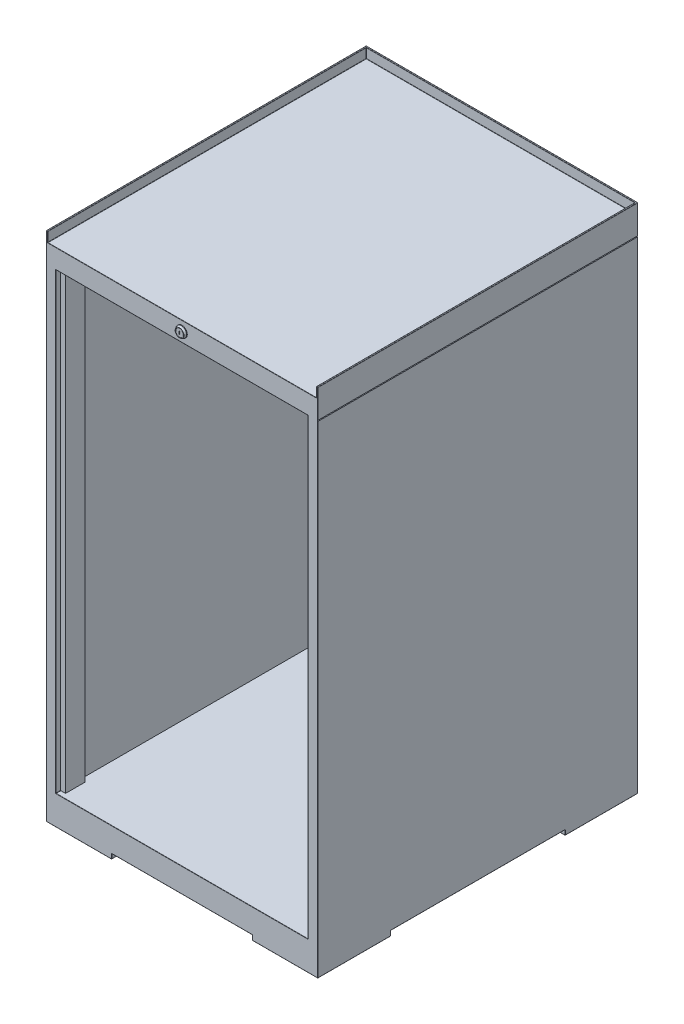
SolidWorks part; units mm, degrees
ref_plane "Frontal" through (0, 0, 0) normal (0, 0, 1) x (1, 0, 0)
ref_plane "Superior" through (0, 0, 0) normal (0, 1, 0) x (1, 0, 0)
ref_plane "Direito" through (0, 0, 0) normal (1, 0, 0) x (0, 0, -1)
sketch "Sketch1" plane through (0, 0, 0) normal (0, 0, 1) x (1, 0, 0)
  line L1 (-280, 527.5) -> (280, 527.5)
  line L2 (-280, 527.5) -> (-280, -527.5)
  line L3 (-280, -527.5) -> (280, -527.5)
  line L4 (280, 527.5) -> (280, -527.5)
  line L5 (-280, 527.5) -> (280, -527.5) construction
  line L6 (-280, -527.5) -> (280, 527.5) construction
  point P0 (0, 0)
  dimension "D1" = 560
  dimension "D2" = 1055
extrude "Boss-Extrude1" add sketch "Sketch1" along normal blind 660
sketch "Sketch2" plane through (0, 0, 660) normal (0, 0, 1) x (1, 0, 0)
  line L0 (280, 527.5) -> (-280, 527.5) construction
  line L1 (-277, 547.5) -> (277, 547.5)
  line L2 (-277, 547.5) -> (-277, 507.5)
  line L3 (-277, 507.5) -> (277, 507.5)
  line L4 (277, 547.5) -> (277, 507.5)
  line L5 (-277, 547.5) -> (277, 507.5) construction
  line L6 (-277, 507.5) -> (277, 547.5) construction
  line L7 (-280, 527.5) -> (-280, -527.5) construction
  point P0 (0, 527.5)
  dimension "D1" = 3
  dimension "D2" = 20
extrude "Cut-Extrude1" cut sketch "Sketch2" against normal blind 657
sketch "Sketch3" plane through (0, 0, 660) normal (0, 0, 1) x (1, 0, 0)
  line L0 (-277, 507.5) -> (277, 507.5) construction
  line L1 (-260, 467.5) -> (260, 467.5)
  line L2 (-260, 467.5) -> (-260, -467.5)
  line L3 (-260, -467.5) -> (260, -467.5)
  line L4 (260, 467.5) -> (260, -467.5)
  line L5 (-260, 467.5) -> (260, -467.5) construction
  line L6 (-260, -467.5) -> (260, 467.5) construction
  line L7 (-280, 527.5) -> (-280, -527.5) construction
  point P0 (0, 0)
  dimension "D1" = 40
  dimension "D2" = 20
extrude "Cut-Extrude2" cut sketch "Sketch3" against normal blind 657
sketch "Sketch4" plane through (0, -527.5, 0) normal (0, -1, 0) x (1, 0, 0)
  line L0 (-145, 660) -> (-145, 510)
  line L1 (-280, 660) -> (280, 660) construction
  line L2 (-145, 510) -> (-280, 510)
  line L3 (-280, 660) -> (-280, 0) construction
  line L4 (-280, 510) -> (-280, 150)
  line L5 (-280, 150) -> (-145, 150)
  line L6 (-145, 150) -> (-145, 0)
  line L7 (-280, 0) -> (280, 0) construction
  line L8 (-145, 0) -> (145, 0)
  line L9 (145, 0) -> (145, 150)
  line L10 (145, 150) -> (280, 150)
  line L11 (280, 660) -> (280, 0) construction
  line L12 (280, 150) -> (280, 510)
  line L13 (280, 510) -> (145, 510)
  line L14 (145, 510) -> (145, 660)
  line L15 (145, 660) -> (-145, 660)
  dimension "D1" = 135
  dimension "D2" = 150
  dimension "D3" = 150
  dimension "D4" = 135
extrude "Cut-Extrude3" cut sketch "Sketch4" against normal blind 10
fillet "Filete1" radius 1 2 edges at (278.5, 527.5, 660) (-278.5, 527.5, 660)
sketch "Sketch5" plane through (0, -467.5, 0) normal (0, 1, 0) x (1, 0, 0)
  line L0 (-260, -3) -> (-260, -660) construction
  line L1 (-260, -650) -> (-250, -650)
  line L2 (-260, -650) -> (-260, -610)
  line L3 (-260, -610) -> (-250, -610)
  line L4 (-250, -650) -> (-250, -610)
  line L5 (260, -3) -> (260, -660) construction
  line L6 (260, -650) -> (250, -650)
  line L7 (260, -650) -> (260, -610)
  line L8 (260, -610) -> (250, -610)
  line L9 (250, -650) -> (250, -610)
  line L10 (-260, -660) -> (260, -660) construction
  line L11 (-260, -3) -> (260, -3) construction
  line L12 (-260, -13) -> (-250, -13)
  line L13 (-260, -13) -> (-260, -53)
  line L14 (-260, -53) -> (-250, -53)
  line L15 (-250, -13) -> (-250, -53)
  line L16 (260, -13) -> (250, -13)
  line L17 (260, -13) -> (260, -53)
  line L18 (260, -53) -> (250, -53)
  line L19 (250, -13) -> (250, -53)
  dimension "D1" = 10
  dimension "D2" = 10
  dimension "D3" = 40
  dimension "D4" = 10
  dimension "D5" = 40
  dimension "D6" = 10
  dimension "D7" = 40
  dimension "D8" = 10
  dimension "D9" = 10
  dimension "D10" = 10
  dimension "D11" = 10
  dimension "D12" = 40
extrude "Boss-Extrude2" add sketch "Sketch5" along normal blind 935
sketch "Sketch6" plane through (0, 0, 660) normal (0, 0, 1) x (1, 0, 0)
  line L0 (279, 467.5) -> (280, 468.5)
  line L1 (280, -527.5) -> (280, 526.5) construction
  line L2 (280, 468.5) -> (280, 466.5)
  line L3 (280, 466.5) -> (279, 467.5)
  line L4 (279, 467.5) -> (280, 467.5) construction
  line L5 (-279, 467.5) -> (-280, 468.5)
  line L6 (-280, 526.5) -> (-280, -527.5) construction
  line L7 (-280, 468.5) -> (-280, 466.5)
  line L8 (-280, 466.5) -> (-279, 467.5)
  line L9 (-279, 467.5) -> (-280, 467.5) construction
  dimension "D1" = 1
  dimension "D2" = 2
  dimension "D3" = 1
extrude "Cut-Extrude4" cut sketch "Sketch6" against normal through all
sketch "Sketch7" plane through (-280, 0, 0) normal (-1, 0, 0) x (0, 0, 1)
  line L0 (0, 468.5) -> (1, 467.5)
  line L1 (0, 467.5) -> (660, 467.5) construction
  line L2 (1, 467.5) -> (0, 466.5)
  line L3 (0, 466.5) -> (0, 468.5)
  dimension "D1" = 1
extrude "Cut-Extrude5" cut sketch "Sketch7" against normal through all
sketch "Sketch9" plane through (0, 0, 660) normal (0, 0, 1) x (1, 0, 0)
  line L0 (-277, 507.5) -> (277, 507.5) construction
  circle A0 centre (0, 487.5) radius 11
  dimension "D2" = 22
  dimension "D1" = 20
extrude "Boss-Extrude3" add sketch "Sketch9" along normal blind 1.5
sketch "Sketch10" plane through (0, 0, 661.5) normal (0, 0, 1) x (1, 0, 0)
  circle A1 centre (0, 487.5) radius 11
  circle A2 centre (0, 487.5) radius 11
  dimension "D1" = 0
extrude "Boss-Extrude4" add sketch "Sketch10" along normal blind 3.5 draft 30
sketch "Sketch11" plane through (0, 0, 665) normal (0, 0, 1) x (1, 0, 0)
  circle A0 centre (0, 487.5) radius 8
  circle A1 centre (0, 487.5) radius 7.75
  dimension "D1" = 16
  dimension "D2" = 15.5
extrude "Cut-Extrude6" cut sketch "Sketch11" against normal blind 5
sketch "Sketch12" plane through (0, 0, 665) normal (0, 0, 1) x (1, 0, 0)
  line L1 (-1, 490.5) -> (1, 490.5)
  line L2 (-1, 490.5) -> (-1, 484.5)
  line L3 (-1, 484.5) -> (1, 484.5)
  line L4 (1, 490.5) -> (1, 484.5)
  line L5 (-1, 490.5) -> (1, 484.5) construction
  line L6 (-1, 484.5) -> (1, 490.5) construction
  point P0 (0, 487.5)
  dimension "D1" = 6
  dimension "D2" = 2
extrude "Cut-Extrude7" cut sketch "Sketch12" against normal blind 0.5
fillet "Filete2" radius 0.5 74 edges at (-145, -522.5, 660) (-280, -522.5, 510) (0, -517.5, 660) (-145, -522.5, 0) (0, 527.5, 3) (-212.5, -517.5, 510) (145, -517.5, 585) (280, -517.5, 330) (212.5, -517.5, 150) (-145, -517.5, 75) (280, 527.5, 329.5) (280, 527.2071, 659.7071) (277, 527.5, 331) (277, 527.2071, 659.7071) (-277, 527.5, 331) (-277, 527.2071, 659.7071) (-280, 527.5, 329.5) (-280, 527.2071, 659.7071) (-280, -527.5, 75) (-212.5, -527.5, 150) (-145, -527.5, 75) (-212.5, -527.5, 0) (212.5, -527.5, 0) (145, -527.5, 75) (212.5, -527.5, 150) (280, -527.5, 75) (280, -527.5, 585) (212.5, -527.5, 510) (145, -527.5, 585) (212.5, -527.5, 660) (-212.5, -527.5, 660) (-145, -527.5, 585) (-212.5, -527.5, 510) (-280, -527.5, 585) (-145, -522.5, 510) (-145, -517.5, 585) (145, -522.5, 660) (145, -522.5, 510) (212.5, -517.5, 510) (280, -522.5, 510) (280, -522.5, 150) (145, -522.5, 150) (145, -517.5, 75) (145, -522.5, 0) (0, -517.5, 0) (-145, -522.5, 150) (-212.5, -517.5, 150) (-280, -517.5, 330) (-280, -522.5, 150) (-280, -30.5, 0) (-280, 498, 0) (-280, -30.5, 660) (280, -30.5, 660) (280, -30.5, 0) (280, 498, 0) (0, 527.5, 0) (277, 517.5, 3) (0, 507.5, 3) (-277, 517.5, 3) (-277, 507.5, 331.5) (277, 507.5, 331.5) (280, 497.5, 660) (277, 517, 660) (0, 507.5, 660) (-277, 517, 660) (-280, 497.5, 660) (-260, 467.5, 655) (260, 467.5, 655) (260, -467.5, 655) (-260, -467.5, 655) (0, -467.5, 660) (260, 0, 660) (0, 467.5, 660) (-260, 0, 660)
hole_wizard "Tapped Hole M61" positions "Sketch18" profile "Sketch17" tap size "M6" standard "ISO"
sketch "Sketch18" plane through (0, 0, 0) normal (0, 0, -1) x (-1, 0, 0)
  point P0 (-197.25, 415)
  point P3 (-82.75, 415)
  point P6 (197.25, 415)
  point P9 (82.75, 415)
sketch "Sketch17" plane through (197.25, 415, 0) normal (1, 0, 0) x (0, 1, 0)
  line L0 (0, 0) -> (0, 18.5022)
  line L1 (0, 18.5022) -> (2.5, 17)
  line L2 (2.5, 17) -> (2.5, 0)
  line L5 (2.5, 0) -> (0, 0)
  line L10 (0, 18.5022) -> (-2.5, 17) construction
  line L11 (0, -6.35) -> (0, 107.95) construction
  dimension "Tap Drill Dia." = 5
  dimension "Tap Drill Depth" = 17
  dimension "Drill Angle" = 118
cosmetic thread "Hole Thread17" parameters "D1"=3, "D2"=6
cosmetic thread "Hole Thread18" parameters "D1"=3, "D2"=6
cosmetic thread "Hole Thread19" parameters "D1"=3, "D2"=6
cosmetic thread "Hole Thread20" parameters "D1"=3, "D2"=6
